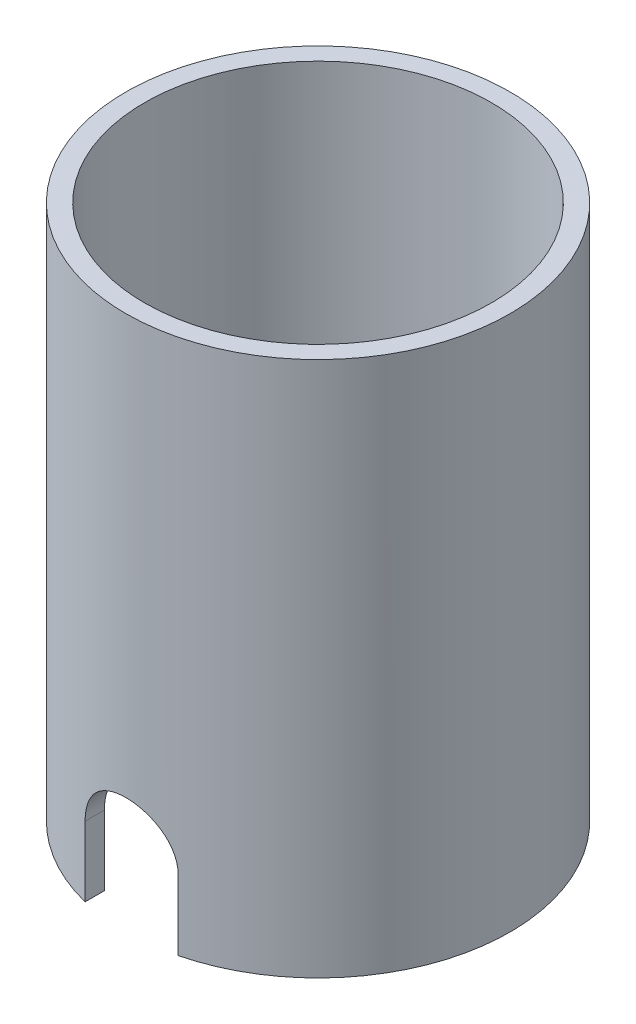
from build123d import *

# Parameters (mm, degrees)
SKETCH1_R               = 82.5
SKETCH1_R_2             = 74.5
BOSS_EXTRUDE1_DEPTH     = 230
CUT_EXTRUDE1_REACH      = 259.9
CUT_EXTRUDE1_END_RADIUS = 82.5


with BuildPart() as part:
    # Sketch1 → Boss-Extrude1 (new body)
    with BuildSketch(Plane(origin=(0, 0, 0), x_dir=(1, 0, 0), z_dir=(0, 1, 0))):
        with Locations(Location((0, 0, 0), (0, 0, 270))):
            Circle(SKETCH1_R)
        with Locations(Location((0, 0, 0), (0, 0, 270))):
            Circle(SKETCH1_R_2, mode=Mode.SUBTRACT)
    extrude(amount=BOSS_EXTRUDE1_DEPTH)

    # Cut-Extrude1: up to this cylinder (the profile starts inside it)
    cut_extrude1_end = Plane(origin=(0, 15, 0), z_dir=(0, -1, 0)) * Cylinder(CUT_EXTRUDE1_END_RADIUS, 685.8, mode=Mode.PRIVATE)
    # Sketch2 → Cut-Extrude1 (cut, up to the surface)
    with BuildSketch(Plane.XY, mode=Mode.PRIVATE) as cut_extrude1_sk1:
        with BuildLine():
            Line((-20, 0), (-20, 30))
            ThreePointArc((-20, 30), (0, 50), (20, 30))
            Line((20, 30), (20, 0))
            ThreePointArc((20, 0), (0, -20), (-20, 0))
        make_face()
    cut_extrude1_tool1 = extrude(cut_extrude1_sk1.sketch, amount=CUT_EXTRUDE1_REACH, mode=Mode.PRIVATE) & cut_extrude1_end
    add(cut_extrude1_tool1.solids().sort_by_distance((0, 15, 0))[0], mode=Mode.SUBTRACT)


solid = part.part
